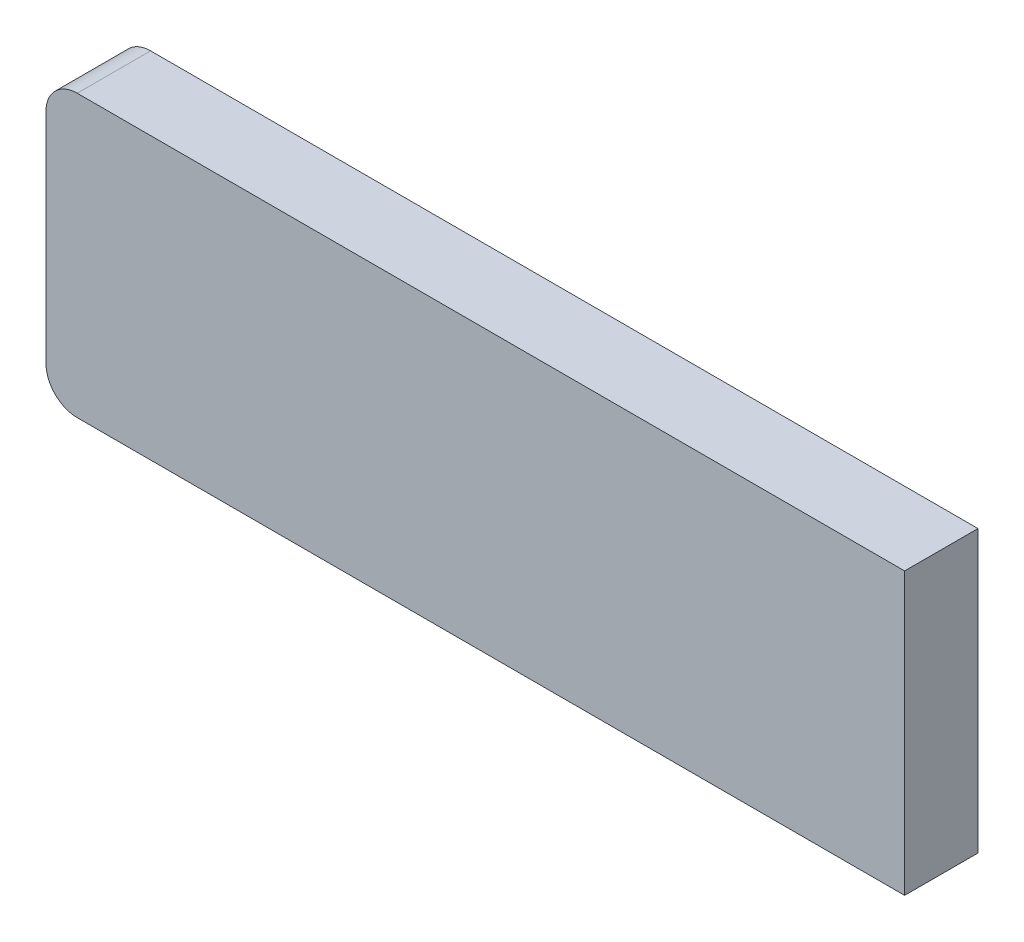
SolidWorks part; units mm, degrees
ref_plane "前视基准面" through (0, 0, 0) normal (0, 0, 1) x (1, 0, 0)
ref_plane "上视基准面" through (0, 0, 0) normal (0, 1, 0) x (1, 0, 0)
ref_plane "右视基准面" through (0, 0, 0) normal (1, 0, 0) x (0, 0, -1)
other "Configuration Table"
sketch "草图1" plane through (0, 0, 0) normal (0, 0, 1) x (1, 0, 0)
  line L1 (-132.5, -45) -> (132.5, -45)
  line L2 (-142.5, -35) -> (-142.5, 35)
  line L3 (-132.5, 45) -> (132.5, 45)
  line L4 (132.5, -45) -> (132.5, 45)
  line L5 (0, 45) -> (0, -45) construction
  line L6 (-142.5, 0) -> (132.5, 0) construction
  arc A0 (-132.5, -45) -> (-142.5, -35) centre (-132.5, -35) cw
  arc A1 (-142.5, 35) -> (-132.5, 45) centre (-132.5, 35) cw
  point P0 (0, 0)
  point P8 (-142.5, 45)
  dimension "D3" = 10
  dimension "D1" = 90
  dimension "D2" = 275
extrude "凸台-拉伸1" add sketch "草图1" along normal blind 23.5
